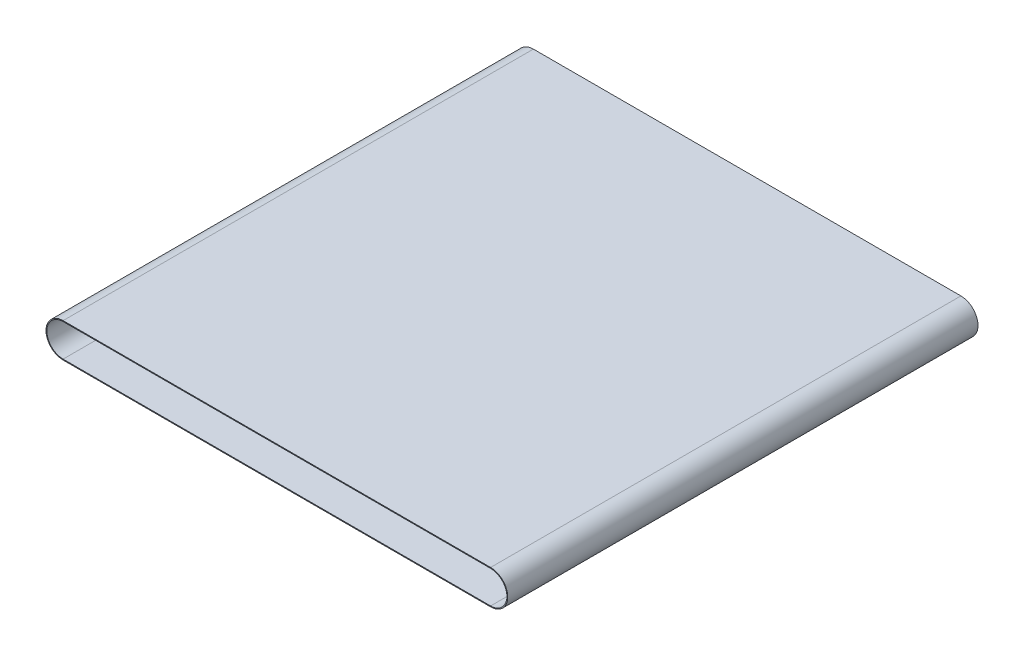
from build123d import *

# Parameters (mm, degrees)
EXTRUDE_1_DEPTH = 550


with BuildPart() as part:
    # 草图1 → 拉伸-薄壁1 (new, symmetric)
    with BuildSketch(Plane.XY):
        with BuildLine():
            Line((500, -40), (-500, -40))
            ThreePointArc((-500, -40), (-540, 0), (-500, 40))
            Line((-500, 40), (500, 40))
            ThreePointArc((500, 40), (540, 0), (500, -40))
        make_face()
        with BuildLine():
            Line((500, -38), (-500, -38))
            ThreePointArc((-500, -38), (-538, 0), (-500, 38))
            Line((-500, 38), (500, 38))
            ThreePointArc((500, 38), (538, 0), (500, -38))
        make_face(mode=Mode.SUBTRACT)
    extrude(amount=EXTRUDE_1_DEPTH, both=True)


solid = part.part
